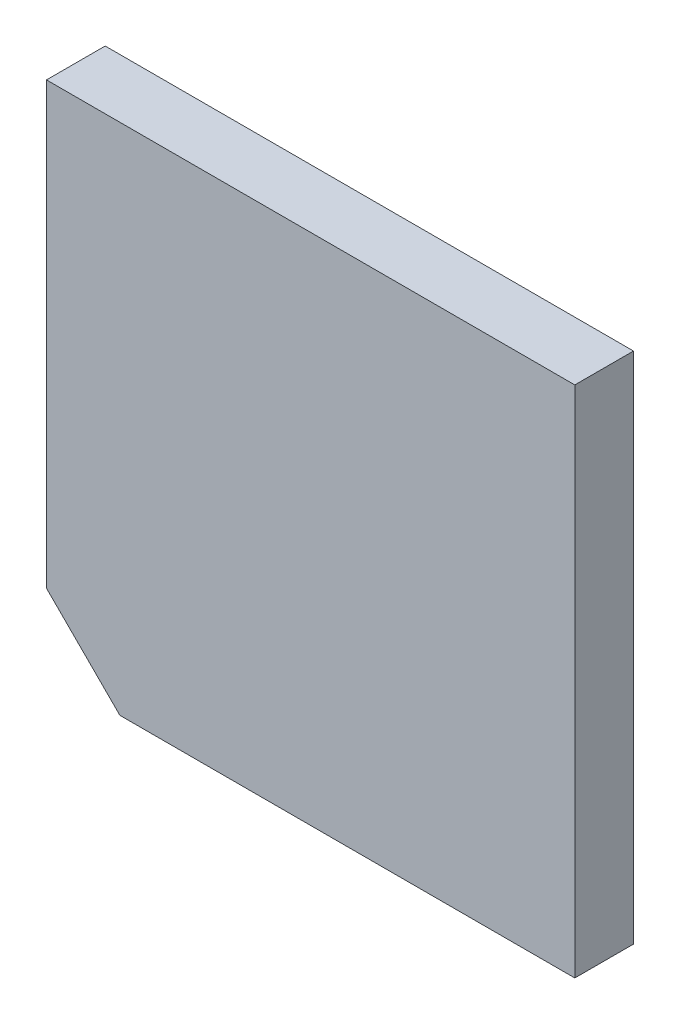
from build123d import *

# Parameters (mm, degrees)
SKETCH1_W           = 36
SKETCH1_H           = 35
BOSS_EXTRUDE1_DEPTH = 4
CHAMFER1_SIZE       = 5


with BuildPart() as part:
    # Sketch1 → Boss-Extrude1 (new body)
    with BuildSketch(Plane.XY):
        with Locations((18, 17.5)):
            Rectangle(SKETCH1_W, SKETCH1_H)
    extrude(amount=BOSS_EXTRUDE1_DEPTH)

    # Chamfer1
    chamfer1_edges = [part.edges().sort_by_distance(p)[0] for p in [
        (0, 0, 2),
    ]]
    chamfer(chamfer1_edges, length=CHAMFER1_SIZE)


solid = part.part
